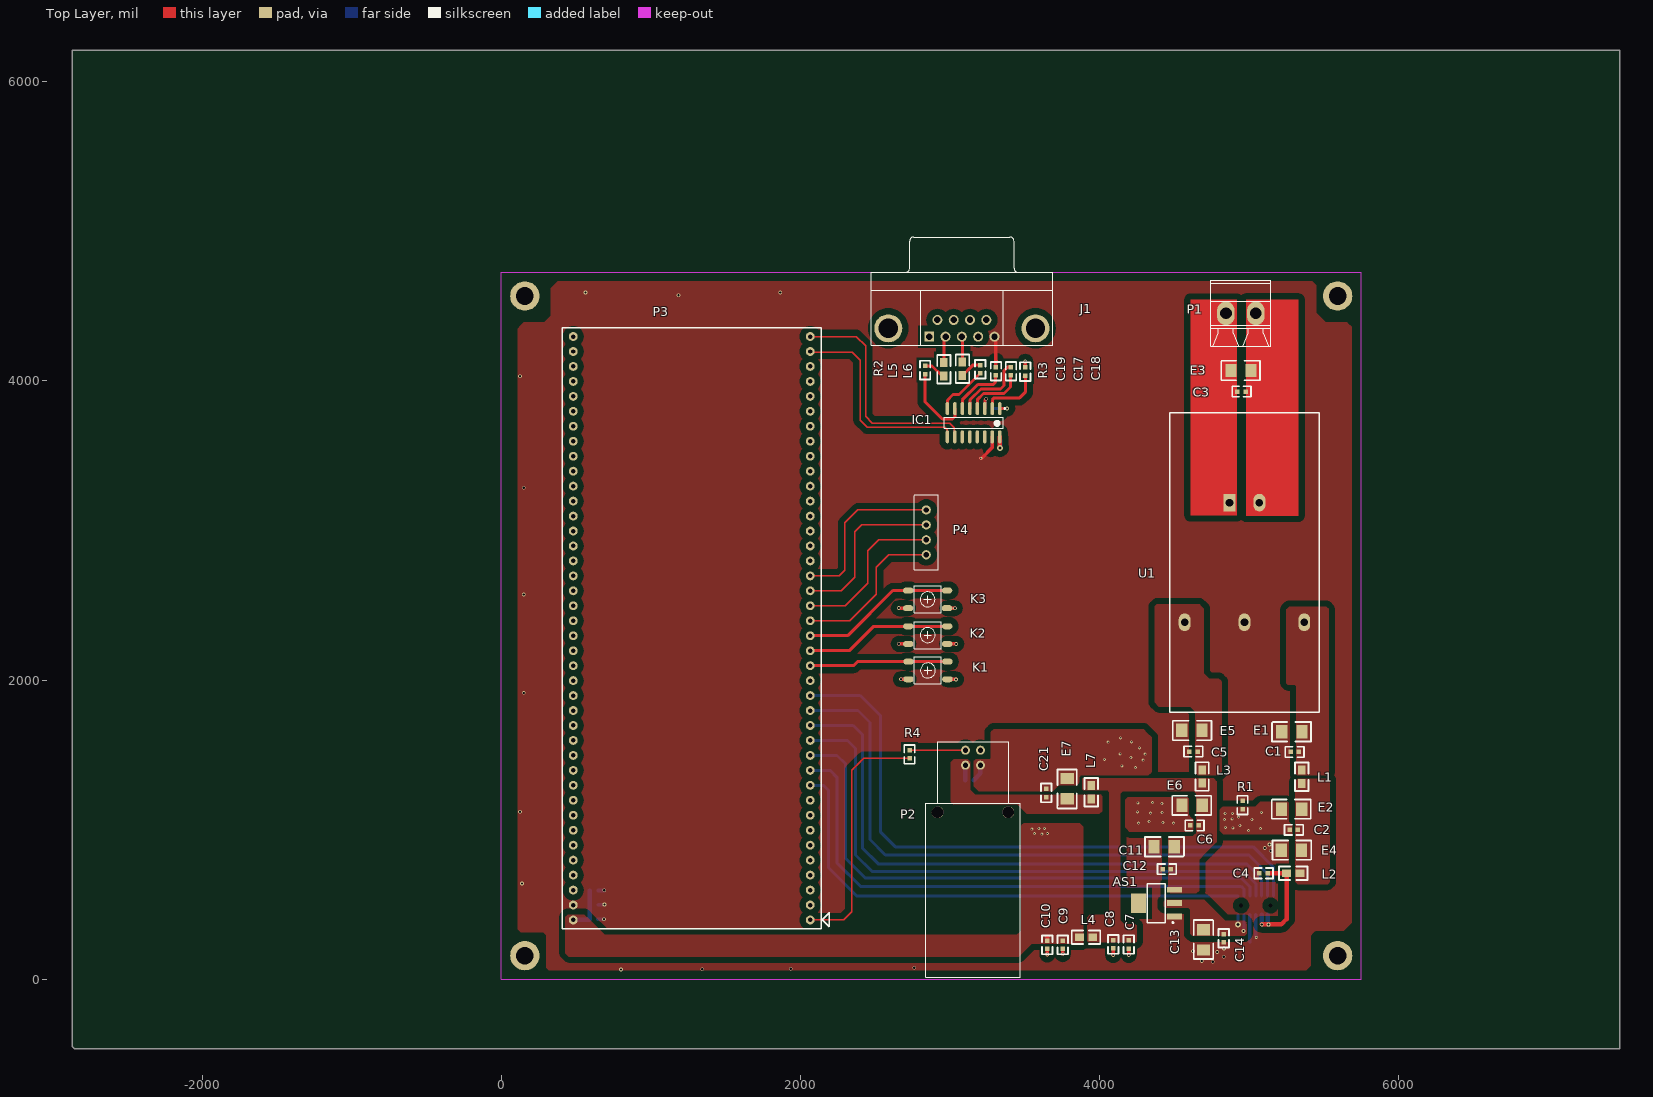
[diagram p0: Top Layer view]
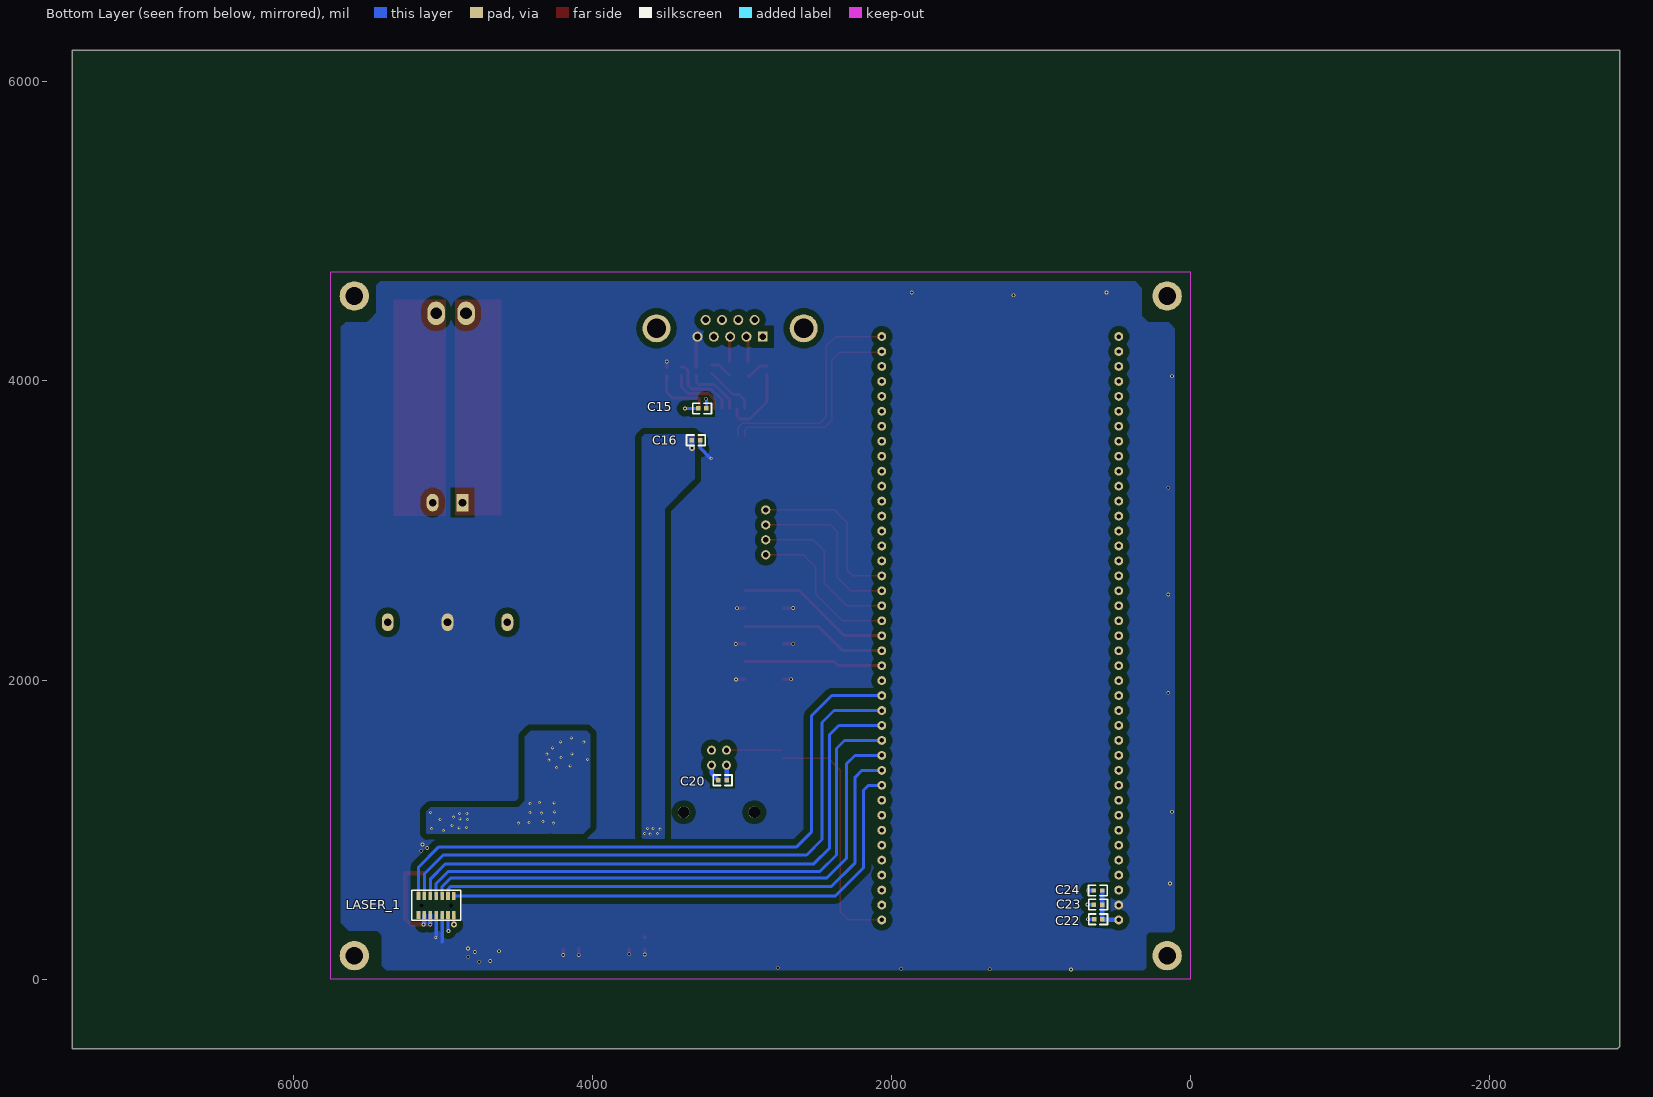
[diagram p1: Bottom Layer view, seen from below]
# Altium PCB MISC79012.PcbDoc
Units mil, origin at the board's own origin, x right, y up, seen from the top; angles counter-clockwise.
Board outline 10345 x 6675 mil, 2 copper layers (Top Layer, Bottom Layer); 54 components, 42 nets, 244 pads, 84 vias.

## Layer stack, top to bottom (the 12.6 mil dielectric is the usual default, probably not edited)
Top Layer: signal copper 1.4
Dielectric: core 12.6, FR-4, Dk 4.8
Bottom Layer: signal copper 1.4

## Board outline
-2868.35,6210 -2868.35,2355 -2868.35,-450 -2853.35,-465 7476.65,-465 7476.65,6210 -2868.35,6210

## Design rules (kind name [scope] priority, off if disabled: settings)
Clearance [All] p1: gap=10
ComponentClearance [All] p1 off: gap=10 collisioncheckmode=3 verticalgap=10 showdistances=FALSE
FabricationTestPointUsage TestPointUsage [All] p1: valid=0 allowmultiple=FALSE
FabricationTestpoint Testpoint [(IsPad And (OnTopLayer Or OnBottomLayer))] p1: side=3 testpointundercomponent=TRUE minsize=40 maxsize=100 preferedsize=60 minholesize=0 maxholesize=40 preferedholesize=32 testpointgrid=1 allowsidetop=TRUE allowsidebottom=TRUE usegrid=TRUE gridtolerance=0.01
HoleSize [All] p1 off: absolutevalues=TRUE maxlimit=100 minlimit=1 maxpercent=80.000 minpercent=20.000
PlaneConnect PlaneConnect_1 [(InPadClass('All Pads'))] p1: planeconnectstyle=Relief reliefexpansion=20 reliefentries=4 reliefconductorwidth=10 reliefairgap=10
PlaneConnect [All] p2: planeconnectstyle=Direct reliefexpansion=20 reliefentries=4 reliefconductorwidth=20 reliefairgap=20
PolygonConnect PolygonConnect_1 [(InPadClass('All Pads'))] p1: connectstyle=Direct reliefconductorwidth=20 reliefentries=4 polygonreliefangle="90 Angle"
PolygonConnect [All] p2: connectstyle=Direct reliefconductorwidth=10 reliefentries=4 polygonreliefangle="90 Angle"
RoutingVias [All] p1: holewidth=10 width=18 viastyle="Through Hole" minholewidth=10 minwidth=18 maxholewidth=15 maxwidth=25
SilkscreenOverComponentPads [All] p1: minsilkscreentomaskgap=10
SolderMaskExpansion SolderMaskExpansion_1 [IsVia] p1: expansion=-40
SolderMaskExpansion [All] p2: expansion=2
Width [All] p1: maxlimit=200 minlimit=8 preferedwidth=10 minimp=50.000000 maximp=50.000000 favimp=50.000000
22 further rules are at their usual default settings.

## Classes and differential pairs
component class MCU-1: C15 C16 C17 C18 C19 C20 C21 C22 C23 C24 C31 C32 C33 E7 IC1 J1 K1 K2 K3 L5 L6 L7 L8 LASER_1 P2 P3 P4 R2 R3 R4
component class LD-1: AS1 C1 C2 C3 C4 C5 C6 C7 C8 C9 C10 C11 C12 C13 C14 E1 E2 E3 E4 E5 E6 L1 L2 L3 L4 P1 R1 U1

## Components (designator, comment, footprint, x,y, rotation, side; value= is the part's Value field where it differs from the comment)
AS1 "AS117" SOT223-4 4379,508 r180 top
C1 "0.1u" 0603 5303,1519 r180 top
C2 "0.1u" 0603 5298,998 r180 top
C3 "0.1u" 0603 4948,3928 r0 top
C4 "0.1u" 0603 5095,708 r180 top
C5 "0.1u" 0603 4627,1522 r180 top
C6 "0.1u" 0603 4634,1028 r180 top
C7 "0.1U" 0603 4195,232 r90 top
C8 "0.1U" 0603 4090,233 r90 top
C9 "0.1U" 0603 3753,230 r90 top
C10 "0.1u" 0603 3650,230 r270 top
C11 "10u" 1210 4431,885 r0 top
C12 "0.1u" 0603 4449,736 r180 top
C13 "10u" 1210 4694,263 r90 top
C14 "0.1u" 0603 4830,274 r270 top
C15 "100n/50V" 0603 3265.65,3815.49 r180 bottom
C16 "100n/50V" 0603 3307,3603 r0 bottom
C17 "100n/50V" 0603 3406.65,4064 r90 top
C18 "100n/50V" 0603 3502.65,4062 r270 top
C19 "100n/50V" 0603 3306.65,4064 r270 top
C20 "0.1u" 0603 3129.65,1330 r0 bottom
C21 "0.01u" 0603 3643,1245 r90 top
C22 "0.1U" 0603 618.65,400 r180 bottom
C23 "0.1U" 0603 619.15,499 r180 bottom
C24 "0.1U" 0603 619.65,593 r180 bottom
E1 "22U" 1210 5284.65,1654 r180 top
E2 "22U" 1210 5282.65,1137 r180 top
E3 "22U" 1210 4944.65,4069 r180 top
E4 "22U" 1210 5281.65,863 r0 top
E5 "22U" 1210 4615.65,1663 r0 top
E6 "22U" 1210 4617.65,1162 r180 top
E7 "10U" 1210 3782,1274 r270 top
IC1 "MAX3232" SOIC127P600-16N 3157,3720 r270 top
J1 "D Connector 9" DSUB1.385-2H9 3078.65,4725 r0 top
K1 "KFC-006S-HN" KNOB-SMD 2852,2064 r180 top
K2 "KFC-006S-HN" KNOB-SMD 2850.65,2300 r180 top
K3 "KFC-006S-HN" KNOB-SMD 2849.65,2539 r180 top
L1 "1UH" 0805 5350.65,1353 r270 top
L2 "1UH" 0805 5294,708 r180 top
L3 "1UH" 0805 4684.65,1355 r270 top
L4 "1UH" 0805 3908.65,280.5 r0 top
L5 "600Ω/500mA-0805" 0805 2958.65,4078 r90 top
L6 "600Ω/500mA-0805" 0805 3082.65,4081 r90 top
L7 "1UH" 0805 3943,1250 r270 top
LASER_1 "1905LMIC" CLM-107-02-H-D-K-TR 4998.65,503 r180 bottom
P1 "" MKDS3_2RMI 4943.65,4451 r90 top
P2 "PD" guang2 2916.65,1116 r90 top
P3 "Header 10X2" c8051 1272.65,2346 r90 top
P4 "Header 4H" DIP-4 2840.65,2837 r180 top
R1 "0R" 0603 4955,1164 r90 top
R2 "100" 0603 2833,4072 r270 top
R3 "100" 0603 3202,4077 r270 top
R4 "0R" 0603 2729,1503 r90 top
U1 "YD10" YD10 4967.65,2786 r270 top

## Footprints (in the part's own frame and the unit in brackets; to place one, negate y for a bottom-side part, rotate by r counter-clockwise, add the part's x,y. Pads: shape width x height; smd on the part's side, far side on the other; paste and mask are expansions set on the pad)
0603 [mil]
  rect 30x30 smd: 1(-27.5,0) 2(27.5,0)
  silkscreen extent -63,-35 63,35
0805 [mil]
  rect 60x50 smd: 1(-45,0) 2(45,0)
  silkscreen extent -95,-45 95,45
1210 [mil]
  rect 75x90 smd: 1(67.5,0) 2(-67.5,0)
  silkscreen extent -128,-65 132,65
c8051 [mil]
  oval 59.21x59.06 hole 30: 1(-1950,-792) 2(-1850,-792) 3(-1750,-792) 4(-1650,-792) 5(-1550,-792) 6(-1450,-792) 7(-1350,-792) 8(-1250,-792) 9(-1150,-792) 10(-1050,-792) 11(-950,-792) 12(-850,-792) 13(-750,-792) 14(-650,-792) 15(-550,-792) 16(-450,-792) 17(-350,-792) 18(-250,-792) 19(-150,-792) 20(-50,-792) 21(50,-792) 22(150,-792) 23(250,-792) 24(350,-792) 25(450,-792) 26(550,-792) 27(650,-792) 28(750,-792) 29(850,-792) 30(950,-792) 31(1050,-792) 32(1150,-792) 33(1250,-792) 34(1350,-792) 35(1450,-792) 36(1550,-792) 37(1650,-792) 38(1750,-792) 39(1850,-792) 40(1950,-792) 41(1950,792) 42(1850,792) 43(1750,792) 44(1650,792) 45(1550,792) 46(1450,792) 47(1350,792) 48(1250,792) 49(1150,792) 50(1050,792) 51(950,792) 52(850,792) 53(750,792) 54(650,792) 55(550,792) 56(450,792) 57(350,792) 58(250,792) 59(150,792) 60(50,792) 61(-50,792) 62(-150,792) 63(-250,792) 64(-350,792) 65(-450,792) 66(-550,792) 67(-650,792) 68(-750,792) 69(-850,792) 70(-950,792) 71(-1050,792) 72(-1150,792) 73(-1250,792) 74(-1350,792) 75(-1450,792) 76(-1550,792) 77(-1650,792) 78(-1750,792) 79(-1850,792) 80(-1950,792)
  silkscreen extent -2008,-920 2008,866
CLM-107-02-H-D-K-TR [mm]
  rect 0.61x1.37 smd mask+0.05: 1(1.857,-1.854) 2(1.857,1.346) 3(0.857,-1.854) 4(0.857,1.346) 5(-0.143,-1.854) 6(-0.143,1.346) 7(-1.143,-1.854) 8(-1.143,1.346) 9(-2.143,-1.854) 10(-2.143,1.346) 11(-3.143,-1.854) 12(-3.143,1.346) 13(-4.143,-1.854) 14(-4.143,1.346)
  round 0 hole 0.635 unplated: 15(1.357,-0.254) 16(-3.643,-0.254)
  silkscreen extent -5.3,-2.79 3.02,2.29
DIP-4 [mil]
  round 62 hole 35: 1(0,0) 2(0,-100) 3(0,-200) 4(0,-300)
  silkscreen extent -79,-400 79,100
DSUB1.385-2H9 [mm] "Connector; D Subminiature; 9 Position; Right Angle; Pitch 1.385 mm"
  rect 1.69x1.69 hole 1.09: 1(-5.54,-10.92)
  round 1.69 hole 1.09: 2(-2.77,-10.92) 3(0,-10.92) 4(2.77,-10.92) 5(5.54,-10.92) 6(-4.155,-8.08) 7(-1.385,-8.08) 8(1.385,-8.08) 9(4.155,-8.08)
  round 4.76 hole 3.26: 10(-12.495,-9.5) 11(12.495,-9.5)
  silkscreen extent -15.4,-12.4 15.4,6
guang2 [mm]
  round 1.524 hole 0.9: 1(10.54,-4.73) 2(8,-4.73) 3(8,-7.27) 4(10.54,-7.27)
  round 2 hole 2: ""(0,0) ""(0,-12)
  silkscreen extent -28,-14 11.94,2
KNOB-SMD [mil]
  oval 70x40 smd: 1(-130,-59) 2(130,-59) 3(130,59) 4(-130,59)
  silkscreen extent -90,-90 90,90
MKDS3_2RMI [mm]
  oval 4x3 hole 2: 1(0,-2.54) 2(0,2.54)
  silkscreen extent -5.59,-5.08 5.59,5.08
SOIC127P600-16N [mm] "SOIC, 16-Leads, Body 9.9x3.9mm, Pitch 1.27mm, IPC Medium Density"
  oval 2.2x0.6 smd: 1(-2.4,4.445) 2(-2.4,3.175) 3(-2.4,1.905) 4(-2.4,0.635) 5(-2.4,-0.635) 6(-2.4,-1.905) 7(-2.4,-3.175) 8(-2.4,-4.445) 9(2.4,-4.445) 10(2.4,-3.175) 11(2.4,-1.905) 12(2.4,-0.635) 13(2.4,0.635) 14(2.4,1.905) 15(2.4,3.175) 16(2.4,4.445)
  silkscreen extent -2.52,-5 0.9,5.42, body extent -2,-5 2,5, height 1.75
SOT223-4 [mil] "SOT223-4"
  rect 100x40 smd: 1(-120,90) 2(-120,0) 3(-120,-90)
  rect 100x130 smd: 4(120,0)
  silkscreen extent -115,-130 60,135
YD10 [mm]
  rect 3x2 hole 1.3: 1(-10.16,-2.54)
  oval 3x2 hole 1.3: 2(-10.16,2.54) 3(10.16,10.16) 4(10.16,0) 5(10.16,-10.16)
  silkscreen extent -25.4,-12.7 25.4,12.7

## Part data
AS1: library part "Volt Reg", "Voltage Regulator"
C1 C2 C3 C4 C5 C6 C7 C8 C9 C10 C11 C12 C13 C14 C20 C21 C22 C23 C24: library part CAP, "Capacitor"
C15 C16 C17 C18 C19: library part "CAPACITOR NON-POL"
E1 E2 E3 E4 E5 E6 E7: library part "Cap Pol1", "Polarized Capacitor (Radial)"
J1: library part JG
K1 K2 K3: library part KNOB-SMD
L1 L2 L3 L4 L7: library part INDUCTOR
L5 L6: library part BEAD
LASER_1: library part 1905LMI
P1 P2: library part "Header 7", "Header, 7-Pin"
P3: "Header, 10-Pin, Dual row"
P4: "Header, 4-Pin, Right Angle"
R1 R4: library part RES1
R2 R3: library part SMDRXX_2

## Free pads (board coordinates)
  round 196.85 hole 118.11: 0(157.48,157.48) 0(157.48,4566.93) 0(5590.55,157.48) 0(5590.55,4566.93)

## Via types
v1: diameter 25, hole 15, Top Layer to Bottom Layer, 41 vias
v2: diameter 20, hole 10, Top Layer to Bottom Layer, 39 vias
v3: diameter 18, hole 10, Top Layer to Bottom Layer, 2 vias
v4: diameter 40, hole 20, Top Layer to Bottom Layer, 2 vias

## Nets (pads, with @x,y where several pads share a name; then routed paths per layer and width w, separated by ;. In a path a pad name is that pad's centre, name@x,y a point inside that pad or via, vN(x,y) a via of type N, cw(c..) or ccw(c..) an arc to the next point about the centre after c; other vN are vias at no path point)
3.3V: AS1.2 C13.1 C14.1 LASER_1.1 LASER_1.3 | length 175.9
  Bottom Layer w20: v4@4925.54,365.46 LASER_1.1 ; v1(4962,322) 4964.52,322 4964.91,322.39 LASER_1.3
  Bottom Layer w30: v4@4925.54,365.46 v4(4926,365)
5VD_MCU: C9.2 C10.1 C16.2 C22.2 C23.2 C24.2 IC1.16 L4.1 P3.80 | length 434.5
  Top Layer w30: v4(3332,3551) IC1.16 ; 3650,279.5 3651,280.5
  Bottom Layer w30: P3.80 587.15,396 591.65,400.5 C23.2 592.15,499.5 C24.2 ; v4(3332,3551) 3334.5,3553.5 C16.2
  other v2: 3613,970 3563,973 3651,974 3547,1004 3593,1008 3631,1009
+5V: AS1.3 C6.1 C7.2 C8.2 C11.1 C12.1 E6.2 L3.2 L4.2 L7.1
+5V1: C5.1 E5.1 L3.1 U1.5
-5V: C2.1 E2.2 E4.1 L1.2 L2.1
-5V1: C1.1 E1.2 L1.1 U1.3
A1N0.0: P3.1 R4.1 | length 1665.1
  Top Layer w10: P3.1 2288,396 2344,452 2344,1397 2422.5,1475.5 R4.1
AGND: C2.2 C6.2 C20.2 C21.2 E2.1 E6.1 E7.2 P2.3 R1.1 | length 119.9
  Bottom Layer w30: C20.2 3202.87,1375.72 P2.3
  other v2: 4995,994 5074,1007 4890,1011 4840,1015 4937,1028 4260,1043 4495,1044 4422,1047 4330,1054 4834,1066 5017,1068 4886,1071 4928,1084 4838,1108 4887,1108 4340,1110 4417,1114 5080,1116 4252,1119 4416,1174 4255,1179 4353,1180 4238,1414 4148,1426 4291,1465 4031,1469 4209,1482 4304,1504 4136,1506 4265,1547 4056,1584 4213,1586 4140,1613
GND: AS1.1 C1.2 C4.2 C5.2 C7.1 C8.1 C9.1 C10.2 C11.2 C12.2 C13.2 C14.2 C16.1 C18.1 C19.1 C22.1 C23.1 C24.1 E1.1 E4.2 E5.2 IC1.15 J1.5 K1.3 K1.4 K2.3 K2.4 K3.3 K3.4 LASER_1.5 LASER_1.7 P3.79 R1.2 U1.4 | length 1547.5
  Top Layer w23.62: v1(2657,2242) 2658,2241 K2.3 ; v1(2657,2481) 2658,2480 K3.3 ; v1(2671,2005) K1.3 ; K3.4 v1(3032,2480) ; K2.4 v1(3041,2241) ; K1.4 3039,2005 v1(3040,2004) ; v3(3206,3483) 3211,3483 3282,3554 IC1.15 ; J1.5 3306.65,4285.19 3306.65,4134.65 ; C19.1 3306.65,4134.65 ; 3307,4135 3306.65,4134.65 ; C18.1 v1(3502.65,4128.65) ; v1(3650,165) C10.2 ; v1(3753,167) C9.1 ; v1(4090,161) C8.1 ; v1(4195,162) C7.1
  Bottom Layer w23.62: C22.1 v1(687,400) ; C23.1 v1(690,499) ; C24.1 687,593 v1(688,594) ; v3(3206,3483) 3211,3483 3279.5,3551.5 C16.1 ; 5002,249 5004.28,251.28 5004.28,371.28 ; 5004,371 5004.28,371.28 ; LASER_1.5 5004.28,371.28 ; LASER_1.7 5043.65,373.35 ; 5044,373 5043.65,373.35 ; v3(5047,279) 5043.65,282.35 5043.65,373.35
  other v1: 800,65 1344,66 1935,70 2761,77 4755,117 4683,122 4829,150 4785,182 4623,187 4831,206 139,639 5143,859 5103,877 5135,901 125,1119 150,1914 150,2572 150,3286 125,4031 1185,4572 563,4590 1864,4590
NetC3_1: C3.1 E3.1 P1.2 U1.1
NetC3_2: C3.2 E3.2 P1.1 U1.2
NetC15_1: C15.1 IC1.1 | length 137.3
  Top Layer w20: IC1.1 3380.49,3814.49 v1(3381,3815)
  Bottom Layer w20: C15.1 3380.51,3815.49 v1(3381,3815)
NetC15_2: C15.2 IC1.3 | length 135.8
  Top Layer w20: IC1.3 3232,3870 v1(3242,3880)
  Bottom Layer w20: C15.2 3238.15,3876.15 v1(3242,3880)
NetC17_1: C17.1 IC1.4 | length 395.3
  Top Layer w20: IC1.4 3182,3874 3224,3916 3361,3916 3403,3958 3403,4032.85 C17.1
NetC17_2: C17.2 IC1.5 | length 481.7
  Top Layer w20: IC1.5 3132,3873 3133,3873 3206,3946 3337,3946 3360,3969 3360,4010 3360,4068 3383.5,4091.5 C17.2
NetC18_2: C18.2 IC1.2 | length 423.2
  Top Layer w20: IC1.2 3282,3873 3295,3886 3465,3886 3502.65,3923.65 C18.2 C18.2@3494,4025.85
NetC19_2: C19.2 IC1.6 | length 376
  Top Layer w20: IC1.6 3082,3873 3185,3976 3289,3976 3304,3991 3304,4033.85 C19.2
NetC20_1: C20.1 C21.1 E7.1 L7.2 P2.2 | length 101.3
  Bottom Layer w30: C20.1 3102.15,1430.24 P2.2
NetIC1_7: IC1.7 R2.2 | length 490.7
  Top Layer w20: R2.2 2833,3860 2948,3745 3015,3745 3032,3762 IC1.7
NetIC1_8: IC1.8 R3.2 | length 349.9
  Top Layer w20: IC1.8 2982,3870 3020,3908 3059,3908 3200.5,4049.5 R3.2
NetJ1_2: J1.2 L5.2 | length 176.6
  Top Layer w20: L5.2 2958.65,4284.13 J1.2
NetJ1_3: J1.3 L6.2 | length 170.7
  Top Layer w20: J1.3 3082.65,4291.08 L6.2
NetK1_1: K1.1 K1.2 P3.18 | length 928.5
  Top Layer w20: P3.18 2355,2096 2382,2123 K1.2 K1.1
NetK2_1: K2.1 K2.2 P3.19 | length 983.5
  Top Layer w20: P3.19 2326,2196 2489,2359 K2.2 K2.1
NetK3_1: K3.1 K3.2 P3.20 | length 1040.1
  Top Layer w20: P3.20 2315,2296 2617,2598 K3.2 K3.1
NetL5_1: L5.1 R2.1 | length 153.9
  Top Layer w20: R2.1 2879.5,4099.5 2946,4033 L5.1 L5.1@2958.15,4033.5
NetL6_1: L6.1 R3.1 | length 147.7
  Top Layer w20: L6.1 3151.15,4104.5 R3.1
NetP3_21: P3.21 P4.1 | length 1064.1
  Top Layer w10: P3.21 2330,2396 2508,2574 2508,2754 2591,2837 P4.1
NetP3_22: P3.22 P4.2 | length 1085.8
  Top Layer w10: P3.22 2299,2496 2449,2646 2449,2863 2523,2937 P4.2
NetP3_23: P3.23 P4.3 | length 1136.7
  Top Layer w10: P3.23 2272,2596 2363,2687 2363,2991 2409,3037 P4.3
NetP3_24: P3.24 P4.4 | length 1144.4
  Top Layer w10: P3.24 2260,2696 2297,2733 2297,3050 2384,3137 P4.4
P1.0: LASER_1.10 P3.14 | length 4000.8
  Bottom Layer w20: P3.14 2352,1696 2413,1635 2413,877 2519,771 4981,771 5083.02,668.98 LASER_1.10
P1.1: LASER_1.8 P3.13 | length 3875.1
  Bottom Layer w20: P3.13 2314,1596 2368,1542 2368,831 2479,720 4963,720 5043.65,639.35 LASER_1.8
P1.2: LASER_1.2 P3.10 | length 3470.8
  Bottom Layer w20: P3.10 2154,1296 2187,1263 2187,745 2376.01,555.99 LASER_1.2
P1.3: LASER_1.4 P3.11 | length 3609.7
  Bottom Layer w20: P3.11 2197,1396 2243,1350 2243,779 2401,621 4946,621 4964.91,602.09 LASER_1.4
P1.4: LASER_1.6 P3.12 | length 3735.4
  Bottom Layer w20: P3.12 2244,1496 2302,1438 2302,807 2431,678 4945,678 5004.28,618.72 LASER_1.6
P1.5: LASER_1.12 P3.15 | length 4117.1
  Bottom Layer w20: P3.15 2384,1796 2464,1716 2464,934 2567,831 4997,831 5122.39,705.61 LASER_1.12
P1.6: LASER_1.14 P3.16 | length 4219.9
  Bottom Layer w20: P3.16 2399,1896 2536,1759 2536,983 2634,885 5026,885 5161.76,749.24 LASER_1.14
PD-: P2.1 R4.2 | length 374.1
  Top Layer w10: R4.2 3102.41,1530.5 P2.1
RX: IC1.9 P3.39 | length 1415.2
  Top Layer w10: P3.39 2068.65,4192 2345,4192 2399,4138 2399,3738 2447,3690 2964,3690 2982,3672 IC1.9
TX: IC1.10 P3.40 | length 1555.2
  Top Layer w10: P3.40 2372,4296 2435,4233 2435,3762 2479,3718 2998,3718 3029,3687 3029,3628.51 IC1.10
VCC-5V: C4.1 L2.2 LASER_1.9 LASER_1.11 | length 743.8
  Top Layer w30: v1(5083,366) 5213,366 5249,402 L2.2 C4.1
  Bottom Layer w30: v1@5083.02,366.02 LASER_1.9 ; LASER_1.11 5122.39,371.61 v1(5128,366)
pads on no net: AS1.4 IC1.11 IC1.12 IC1.13 IC1.14 J1.1 J1.4 J1.6 J1.7 J1.8 J1.9 J1.10 J1.11 LASER_1.13 LASER_1.15 LASER_1.16 P2. P2.4 P3.2 P3.3 P3.4 P3.5 P3.6 P3.7 P3.8 P3.9 P3.17 P3.25 P3.26 P3.27 P3.28 P3.29 P3.30 P3.31 P3.32 P3.33 P3.34 P3.35 P3.36 P3.37 P3.38 P3.41 P3.42 P3.43 P3.44 P3.45 P3.46 P3.47 P3.48 P3.49 P3.50 P3.51 P3.52 P3.53 P3.54 P3.55 P3.56 P3.57 P3.58 P3.59 P3.60 P3.61 P3.62 P3.63 P3.64 P3.65 P3.66 P3.67 P3.68 P3.69 P3.70 P3.71 P3.72 P3.73 P3.74 P3.75 P3.76 P3.77 P3.78

## Polygon pours and split planes (outlines as drawn)
GND on Top Layer "Top Layer-No Net" (solid, remove dead copper, pour order 1006): 109,4125 109,334 124,319 129,314 170,314 281,314 292,303 301,294 301,264 301,76 308,69 318,59 359,59 5380,59 5402,81 5410,89 5410,181 5410,291 5429,310 5444,325 5548,325 5633,325 5654,346 5685,377 5685,458 5685,4360 5656,4389 5654,4391 5617,4391 5511,4391 5490,4412 5448,4454 5448,4541 5448,4639 5421,4666 5302,4666 376,4666 330,4620 330,4533 330,4435 301,4406 286,4391 201,4391 151,4391 130,4370 109,4349 109,4125
AGND on Top Layer "Top Layer-No Net" (solid, remove dead copper, pour order 1005): 3159,1439 3159,1290 3179,1270 3192,1257 3656,1257 3687,1257 3712,1282 3728,1298 3747,1298 3846,1298 3859,1311 3863,1315 3863,1344 3863,1350 3871,1358 3875,1362 3908,1362 4324,1362 4343,1381 4349,1387 4349,1512 4349,1616 4316,1649 4293,1672 3810,1672 3291,1672 3276,1657 3271,1652 3271,1627 3271,1478 3268,1475 3264,1471 3229,1471 3170,1471 3160,1461 3159,1460 3159,1439
AGND on Top Layer "Top Layer-No Net" (solid, remove dead copper, pour order 1004): 4543,1216 4186,1216 4174,1204 4170,1200 4170,1074 4170,1016 4185,1001 4199,987 4581,987 4610,987 4622,999 4625,1002 4625,1053 4625,1068 4609,1084 4594,1099 4594,1115 4594,1209 4589,1214 4587,1216 4543,1216
AGND on Top Layer "Top Layer-No Net" (solid, remove dead copper, pour order 1003): 5268,968 4827,968 4804,991 4802,993 4802,1119 4802,1133 4814,1145 4821,1152 4952,1152 5040,1152 5073,1185 5210,1185 5258,1185 5263,1180 5264,1179 5264,1132 5264,1051 5276,1039 5287,1028 5287,1012 5287,972 5284,969 5283,968 5268,968
5VD_MCU on Top Layer "Top Layer-No Net" (solid, remove dead copper, pour order 1002): 3891,336 3891,1018 3878,1031 3866,1043 3589,1043 3491,1043 3483,1035 3474,1026 3474,945 3474,323 3466,315 3447,296 3395,296 691,296 584,403 555,432 468,432 443,432 430,419 428,417 428,383 428,175 442,161 452,151 528,151 3459,151 3513,205 3545,237 3675,237 3883,237 3891,245 3891,336
+5V on Top Layer "Top Layer-No Net" (solid, remove dead copper, pour order 1001): 3885,1311 3885,1268 3890,1263 3891,1262 3928,1262 4053,1262 4057,1258 4064,1251 4064,1193 4064,450 4057,443 4045,431 4009,431 3935,431 3925,421 3918,414 3918,298 3918,254 3926,246 3948,246 4241,246 4245,250 4247,252 4247,286 4247,359 4239,367 4238,368 4213,368 4163,368 4148,383 4137,394 4137,441 4137,1239 4155,1257 4156,1258 4569,1258 4625,1258 4631,1252 4644,1239 4644,1145 4644,976 4632,964 4623,955 4579,955 4471,955 4461,945 4459,943 4459,921 4459,589 4467,581 4474,574 4501,574 4646,574 4661,589 4665,593 4665,676 4665,800 4707,842 4781,916 4781,1195 4781,1323 4768,1336 4762,1342 4705,1342 3887,1342 3885,1340 3885,1311
3.3V on Top Layer "Top Layer-No Net" (solid, remove dead copper, pour order 1000): 4428,518 4428,489 4437,480 4438,479 4486,479 4589,479 4597,471 4604,464 4604,439 4604,305 4618,291 4928,291 4970,291 4982,303 4982,358 4982,379 4974,387 4970,391 4925,391 4840,391 4812,419 4700,531 4545,531 4441,531 4428,518 4428,505
+5V1 on Top Layer "TopLayer-No Net" (solid, remove dead copper, pour order 1000): 4368,2413 4368,2178 4368,1850 4396,1822 4530,1822 4604,1822 4613,1813 4639,1787 4639,1632 4639,1588 4639,1379 4651,1367 4654,1364 4717,1364 4793,1364 4802,1373 4817,1388 4817,1441 4817,1989 4808,1998 4797,2009 4745,2009 4732,2009 4702,2039 4697,2044 4697,2220 4697,2477 4680,2494 4668,2506 4491,2506 4382,2506 4372,2496 4368,2492 4368,2413
-5V1 on Top Layer "TopLayer-No Net" (solid, remove dead copper, pour order 1001): 5248,2403 5248,1980 5255,1973 5258,1970 5302,1970 5303,1970 5314,1959 5314,1870 5314,1370 5319,1365 5320,1364 5338,1364 5515,1364 5522,1371 5530,1379 5530,1449 5530,2476 5515,2491 5272,2491 5266,2491 5256,2481 5248,2473 5248,2403
NetC20_1 on Top Layer "TopLayer-No Net" (solid, remove dead copper, pour order 1002): 3941,1234 3169,1234 3142,1261 3135,1268 3135,1391 3135,1452 3118,1469 3023,1469 3011,1457 3003,1449 3003,1350 3003,1186 3023,1166 3027,1170 3202,1170 3448,1170 3474,1144 3513,1105 3656,1105 3998,1105 4014,1121 4017,1124 4017,1194 4017,1224 4006,1235 4005,1234 3941,1234
-5V on Top Layer "TopLayer-No Net" (solid, remove dead copper, pour order 1003): 5308,1259 5308,652 5317,643 5324,636 5405,636 5524,636 5534,646 5538,650 5538,1219 5538,1331 5529,1340 5330,1340 5324,1340 5314,1330 5308,1324 5308,1259
GND on Bottom Layer "Top Layer-No Net" (solid, remove dead copper, pour order 1009): 105,4125 105,334 120,319 125,314 166,314 277,314 288,303 297,294 297,264 297,76 304,69 314,59 355,59 5376,59 5398,81 5406,89 5406,181 5406,291 5425,310 5440,325 5544,325 5629,325 5650,346 5681,377 5681,458 5681,4360 5652,4389 5650,4391 5613,4391 5507,4391 5486,4412 5444,4454 5444,4541 5444,4639 5417,4666 5298,4666 372,4666 326,4620 326,4533 326,4435 297,4406 282,4391 197,4391 147,4391 126,4370 105,4349 105,4125
AGND on Bottom Layer "Top Layer-No Net" (solid, remove dead copper, pour order 1008): 4013,1549 4013,1021 4044,990 4062,972 4600,972 5102,972 5107,977 5110,980 5110,1043 5110,1122 5098,1134 5084,1148 5043,1148 4497,1148 4473,1172 4453,1192 4453,1262 4453,1620 4432,1641 4411,1662 4349,1662 4038,1662 4023,1647 4013,1637 4013,1549
5VD_MCU on Bottom Layer "Top Layer-No Net" (solid, remove dead copper, pour order 1007): 3515,1031 3515,945 3520,940 3522,938 3557,938 3661,938 3665,942 3671,948 3671,971 3671,3622 3664,3629 3649,3644 3455,3644 3327,3644 3317,3634 3314,3631 3314,3591 3314,3347 3347,3314 3515,3146 3515,1031

## Keep-outs
Keep-Out Layer:
  lines w3.94: 5748.03,0 0,0 0,4724.41 5748.03,4724.41 5748.03,0.59

## Other copper
Top Layer:
  rectangle net NetC3_2: 4977,3098 5329,4544
  rectangle net NetC3_1: 4607,3100 4917,4543